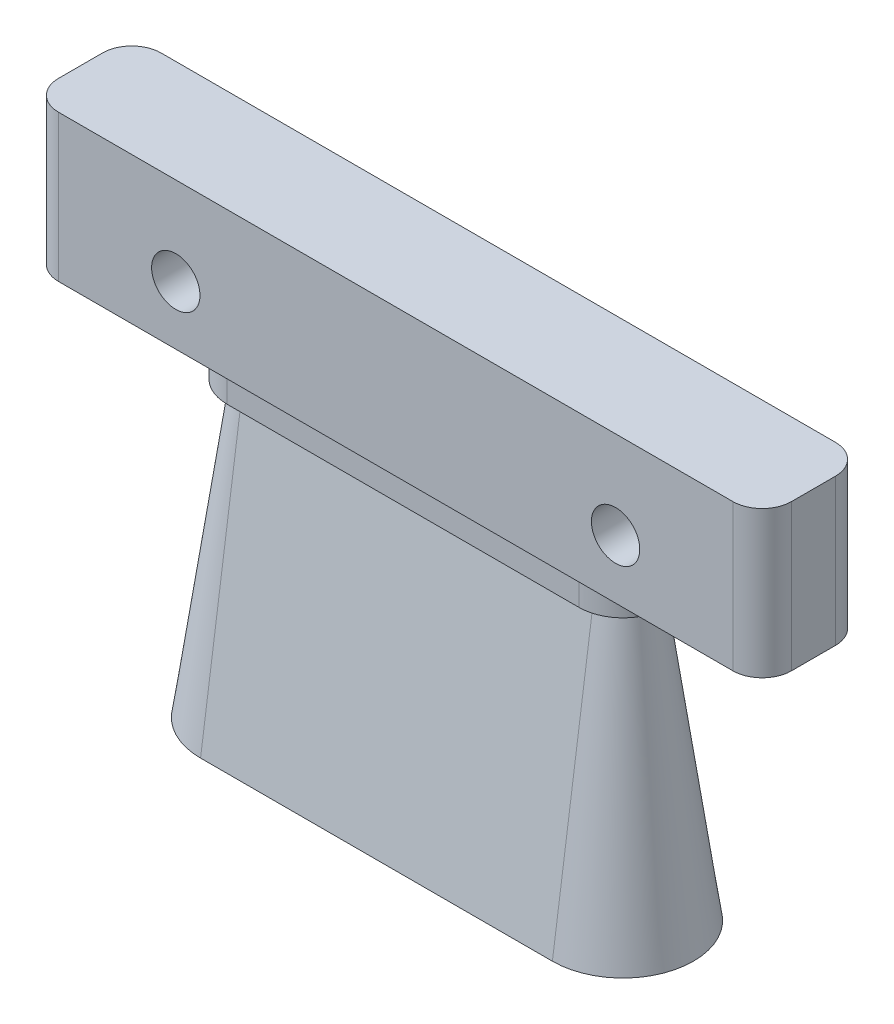
from build123d import *

# Parameters (mm, degrees)
SKETCH_1_3_W          = 50
SKETCH_1_3_H          = 7
BOSS_EXTRUDE1_DEPTH   = 10
BOSS_EXTRUDE2_DEPTH   = 2
BOSS_EXTRUDE3_DEPTH   = 20
BOSS_EXTRUDE3_DRAFT   = -8
FILLET1_R             = 2
M4_TAPPED_HOLE1_D     = 3.3
M4_TAPPED_HOLE1_DEPTH = 10.1
M4_TAPPED_HOLE1_TIP   = 0.991420021


with BuildPart() as part:
    # Sketch 1_3 → Boss-Extrude1 (new body)
    with BuildSketch(Plane(origin=(0, 0, 0), x_dir=(1, 0, 0), z_dir=(0, 1, 0))):
        Rectangle(SKETCH_1_3_W, SKETCH_1_3_H)
    extrude(amount=BOSS_EXTRUDE1_DEPTH)

    # Sketch 1_3 2 → Boss-Extrude2 (add)
    with BuildSketch(Plane(origin=(0, 0, 0), x_dir=(1, 0, 0), z_dir=(0, 1, 0))):
        with BuildLine():
            Line((-12, 3), (12, 3))
            ThreePointArc((12, 3), (15, 0), (12, -3))
            Line((12, -3), (-12, -3))
            ThreePointArc((-12, -3), (-15, 0), (-12, 3))
        make_face()
    extrude(amount=-BOSS_EXTRUDE2_DEPTH)


with BuildPart() as boss_extrude3_tool:
    # Sketch2 → Boss-Extrude3 (with draft: the straight prism first)
    with BuildSketch(Plane.XZ.offset(2)):
        with BuildLine():
            Line((12, 2), (-12, 2))
            ThreePointArc((-12, 2), (-14, 0), (-12, -2))
            Line((-12, -2), (12, -2))
            ThreePointArc((12, -2), (14, 0), (12, 2))
        make_face()
    extrude(amount=BOSS_EXTRUDE3_DEPTH)
    # Boss-Extrude3: the draft: its side faces are tilted about the plane it starts from
    boss_extrude3_sides = [boss_extrude3_tool.faces().sort_by_distance(p)[0] for p in [
        (0, -12, 2),
        (-14, -12, 0),
        (0, -12, -2),
        (14, -12, 0),
    ]]
    draft(boss_extrude3_sides, Plane.XZ.offset(2), BOSS_EXTRUDE3_DRAFT)


with BuildPart() as part_1:
    add(part.part)

    # Boss-Extrude3: add boss_extrude3_tool
    add(boss_extrude3_tool.part)

    # Fillet1
    fillet1_edges = [part_1.edges().sort_by_distance(p)[0] for p in [
        (-25, 5, 3.5),
        (-25, 5, -3.5),
        (25, 5, -3.5),
        (25, 5, 3.5),
    ]]
    fillet(fillet1_edges, radius=FILLET1_R)

    # M4 Tapped Hole1
    with Locations(Plane(origin=(15, 4, -3.5), x_dir=(-1, 0, 0), z_dir=(0, 0, -1))):
        with Locations((0, 0), (30, 0)):
            Hole(M4_TAPPED_HOLE1_D / 2, depth=M4_TAPPED_HOLE1_DEPTH)
            with Locations((0, 0, -(M4_TAPPED_HOLE1_DEPTH + M4_TAPPED_HOLE1_TIP / 2))):  # 118° drill point
                Cone(0, M4_TAPPED_HOLE1_D / 2, M4_TAPPED_HOLE1_TIP, mode=Mode.SUBTRACT)


solid = part_1.part
